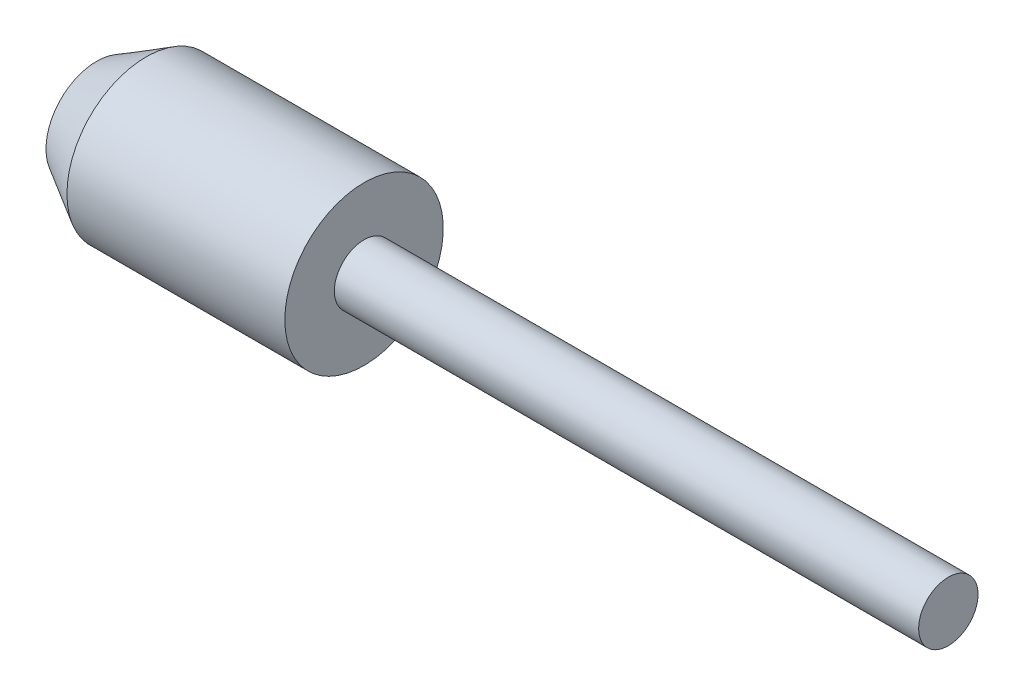
from build123d import *


with BuildPart() as part:
    # Sketch1 → Revolve1 (revolve)
    with BuildSketch(Plane.XY, mode=Mode.PRIVATE) as revolve1_sk:
        Polygon((0, 0), (0, 5.113248654), (5, 8), (27, 8), (27, 3), (86, 3), (86, 0), align=None)
    revolve(revolve1_sk.sketch.rotate(Axis((0, 0, 0), (1, 0, 0)), 90), axis=Axis((0, 0, 0), (1, 0, 0)))


solid = part.part
